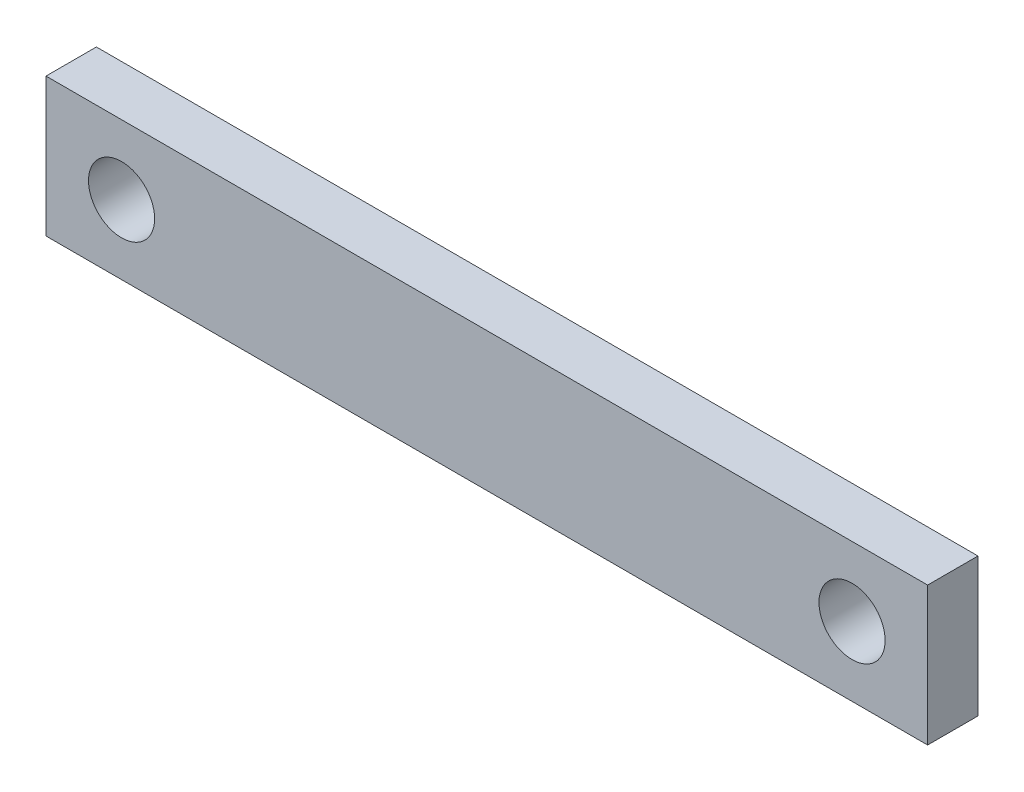
SolidWorks part; units mm, degrees
material "Q235B"
ref_plane "Front Plane" through (0, 0, 0) normal (0, 0, 1) x (1, 0, 0)
ref_plane "Top Plane" through (0, 0, 0) normal (0, 1, 0) x (1, 0, 0)
ref_plane "Right Plane" through (0, 0, 0) normal (1, 0, 0) x (0, 0, -1)
sketch "Sketch1" plane through (0, 0, 0) normal (0, 0, 1) x (1, 0, 0)
  line L1 (-69.9104, 35.003) -> (70.0896, 35.003)
  line L2 (-69.9104, 35.003) -> (-69.9104, 13.003)
  line L3 (-69.9104, 13.003) -> (70.0896, 13.003)
  line L4 (70.0896, 35.003) -> (70.0896, 13.003)
extrude "Boss-Extrude1" add sketch "Sketch1" along normal blind 8
sketch "Sketch2" plane through (0, 0, 8) normal (0, 0, 1) x (1, 0, 0)
  line L0 (0.0896, 13.003) -> (0.0896, 35.003) construction
  line L1 (-69.9104, 13.003) -> (70.0896, 13.003) construction
  line L2 (70.0896, 35.003) -> (-69.9104, 35.003) construction
  circle A0 centre (-57.9104, 24.003) radius 5.25
  circle A1 centre (58.0896, 24.003) radius 5.25
  dimension "D1" = 10.5
  dimension "D2" = 58
  dimension "D3" = 11
extrude "Cut-Extrude1" cut sketch "Sketch2" against normal through all
